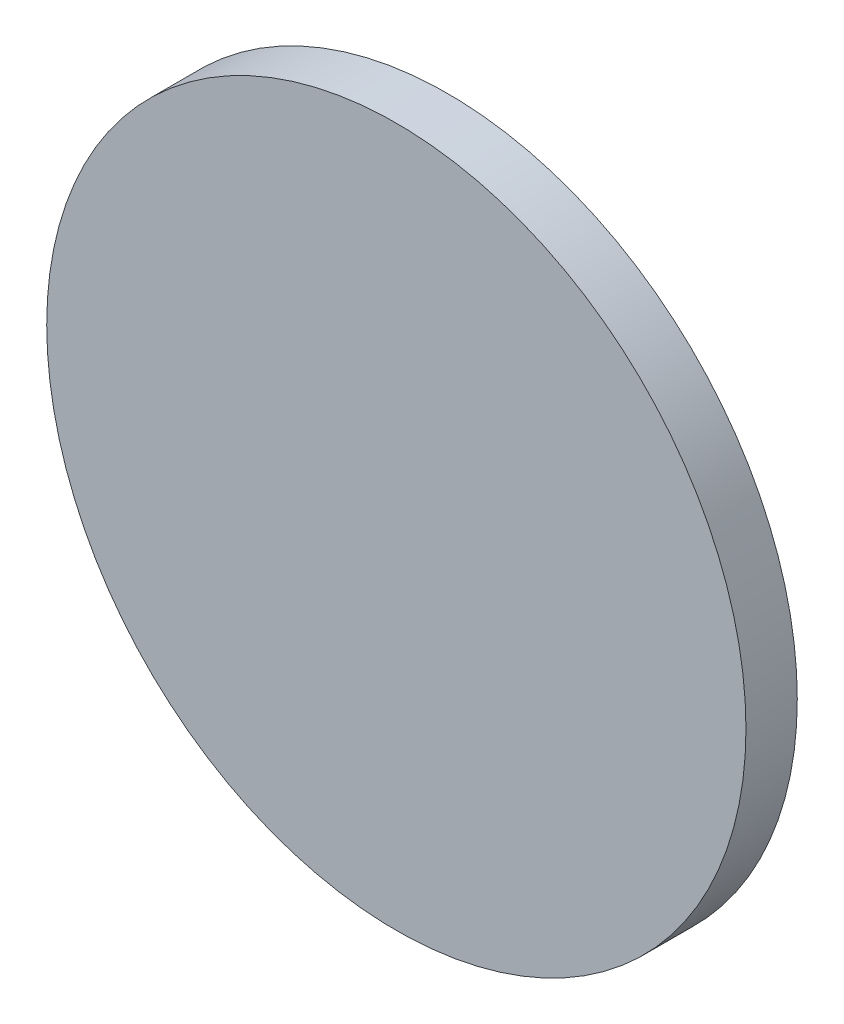
from build123d import *

# Parameters (mm, degrees)
SKETCH_1_R      = 27.25
EXTRUDE_1_DEPTH = 4


with BuildPart() as part:
    # 草图1 → 凸台-拉伸1 (new body)
    with BuildSketch(Plane.XY):
        Circle(SKETCH_1_R)
    extrude(amount=EXTRUDE_1_DEPTH)


solid = part.part
